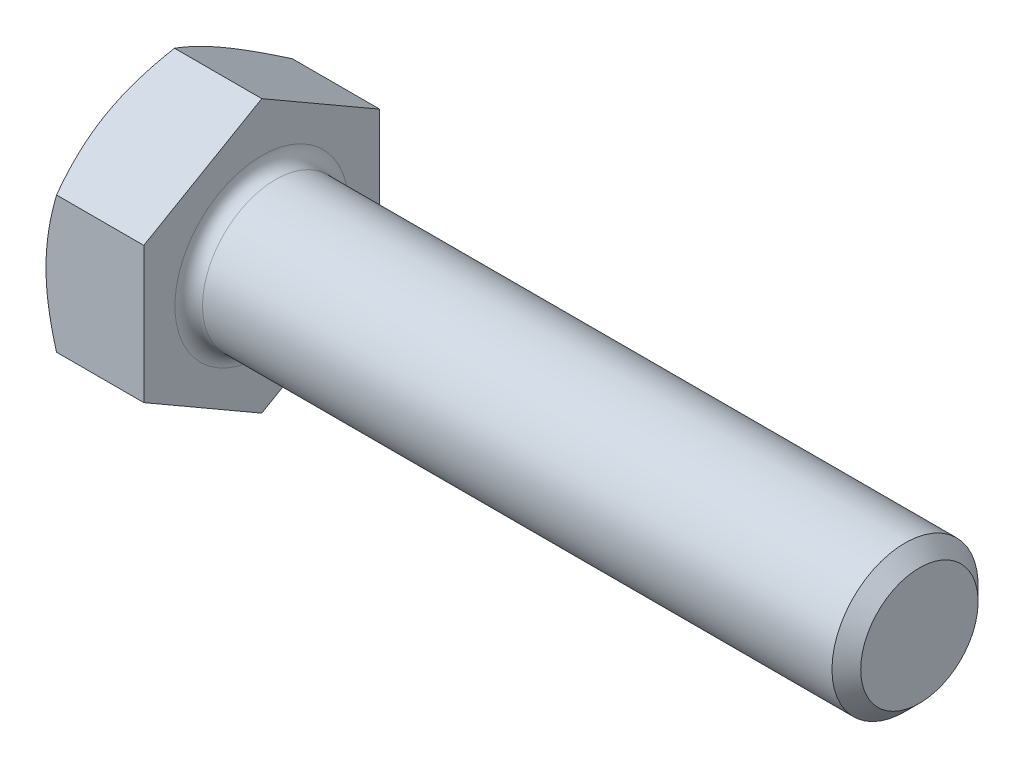
from build123d import *

# Parameters (mm, degrees)
BASE_EXTRUDE_DEPTH = 17
CHAMFER_2_SIZE     = 2.5
FILLET_2_R         = 2.4


with BuildPart() as part:
    # Sketch1 → Base-Extrude (new body)
    with BuildSketch(Plane(origin=(0, 0, 0), x_dir=(0, 0, -1), z_dir=(1, 0, 0))):
        Polygon((20.5, 11.835680518), (20.5, -11.835680518), (0, -23.671361037), (-20.5, -11.835680518), (-20.5, 11.835680518), (0, 23.671361037), align=None)
    extrude(amount=BASE_EXTRUDE_DEPTH)

    # Sketch2 → Boss-Revolve1 (revolve)
    with BuildSketch(Plane.XY, mode=Mode.PRIVATE) as boss_revolve1_sk:
        Polygon((0, 0), (131.3, 0), (131.3, 10.902), (131.3, 12.7), (27.8072, 12.7), (0, 12.7), align=None)
    revolve(boss_revolve1_sk.sketch.rotate(Axis((0, 0, 0), (1, 0, 0)), 90), axis=Axis((0, 0, 0), (1, 0, 0)))

    # Sketch3 → Cut-Revolve1 (revolve, cut)
    with BuildSketch(Plane.XY):
        Polygon((0, 20.5), (4.717737494, 28.671361037), (4.717737494, 33.671361037), (-10, 33.671361037), (-10, 20.5), align=None)
    revolve(axis=Axis((0, 0, 0), (1, 0, 0)), mode=Mode.SUBTRACT)

    # Chamfer 2
    chamfer_2_edges = [part.edges().sort_by_distance(p)[0] for p in [
        (131.3, 0, -12.7),
    ]]
    chamfer(chamfer_2_edges, length=CHAMFER_2_SIZE)

    # Fillet 2
    fillet_2_edges = [part.edges().sort_by_distance(p)[0] for p in [
        (17, 0, -12.7),
    ]]
    fillet(fillet_2_edges, radius=FILLET_2_R)


solid = part.part
